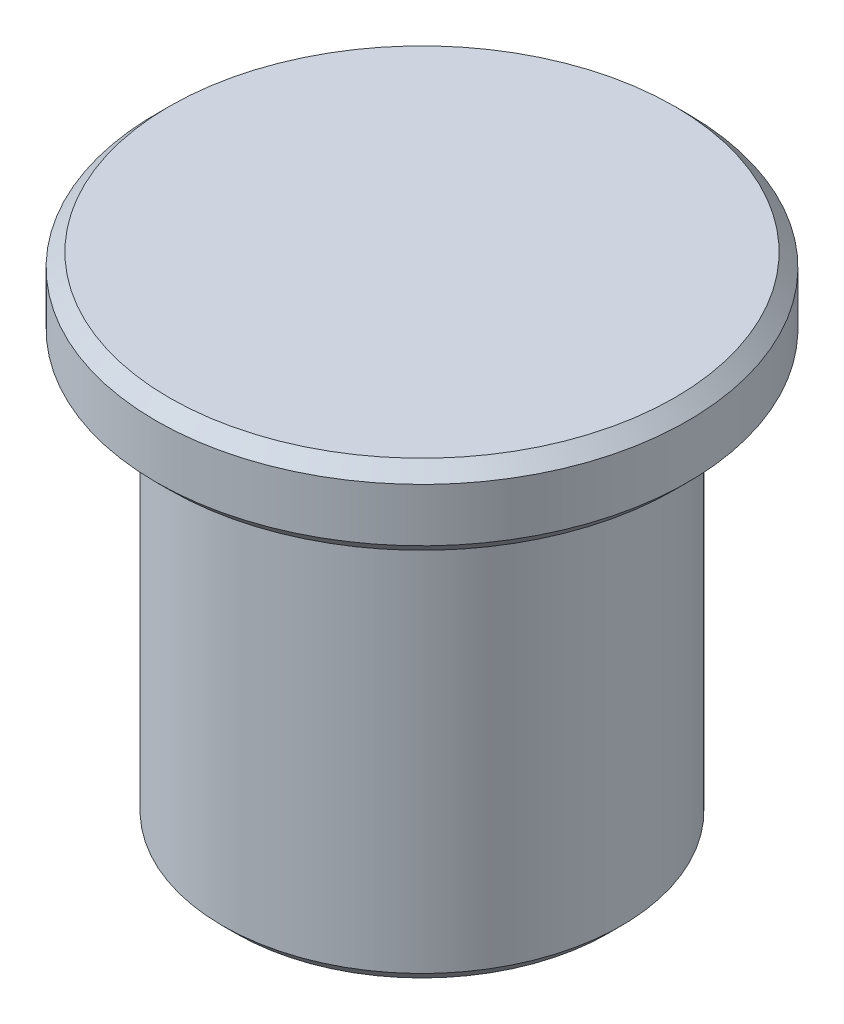
SolidWorks part; units mm, degrees
material "20#"
ref_plane "Front Plane" through (0, 0, 0) normal (0, 0, 1) x (1, 0, 0)
ref_plane "Top Plane" through (0, 0, 0) normal (0, 1, 0) x (1, 0, 0)
ref_plane "Right Plane" through (0, 0, 0) normal (1, 0, 0) x (0, 0, -1)
sketch "Sketch1" plane through (0, 0, 0) normal (0, 0, 1) x (1, 0, 0)
  line L0 (1016.5, 193.3987) -> (1016.5, 219.8987) construction
  line L1 (1010.5, 193.3987) -> (1022.5, 193.3987) construction
  line L2 (762, 219.8987) -> (1222, 219.8987) construction
  line L3 (1009, 204.1987) -> (1009, 219.8987)
  line L4 (1009, 219.8987) -> (1006.5, 219.8987)
  line L5 (1006.5, 219.8987) -> (1006.5, 222.8987)
  line L6 (1006.5, 222.8987) -> (1016.5, 222.8987)
  line L7 (1016.5, 219.8987) -> (1016.5, 222.8987) construction
  line L8 (1016.5, 222.8987) -> (1016.5, 204.1987)
  line L9 (1009, 204.1987) -> (1016.5, 204.1987)
  line L10 (990.5, 204.1987) -> (1122.5, 204.1987) construction
  dimension "D1" = 3
  dimension "D2" = 20
revolve "Revolve1" add sketch "Sketch1" angle 360 about L8
chamfer "Chamfer1" distance 0.5 angle 45 3 edges at (1016.5, 222.8987, 10) (1016.5, 219.8987, 10) (1016.5, 204.1987, 7.5)
